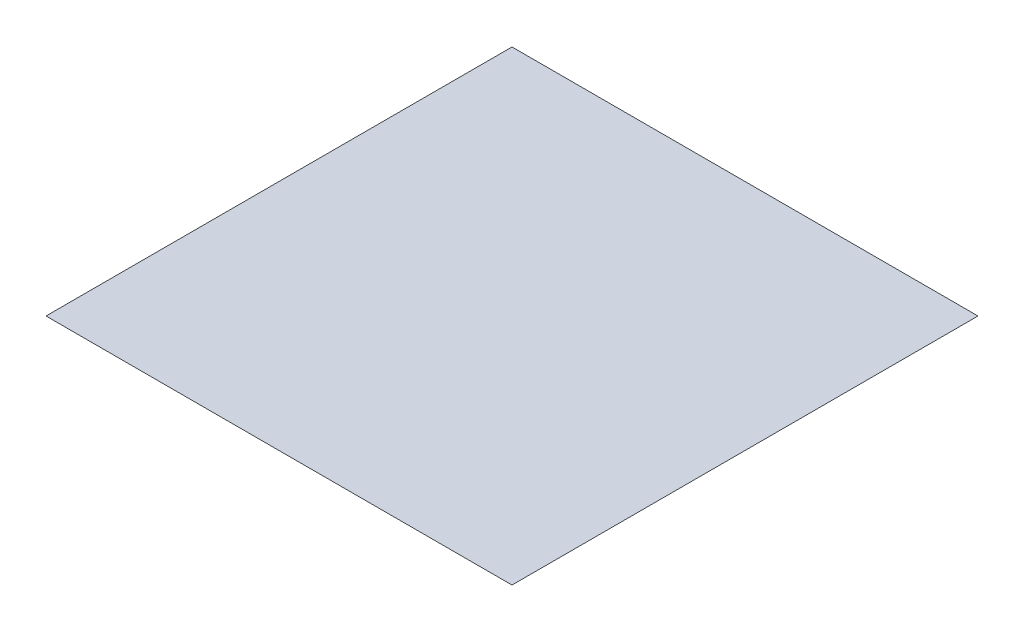
from build123d import *


with BuildPart() as part:
    # 草图5 → 放样1 section 0
    with BuildSketch(Plane(origin=(0, 100, 0), x_dir=(-1, 0, 0), z_dir=(0, -1, 0))):
        with BuildLine():
            Line((165.564800674, -165.564800674), (-165.564800674, -165.564800674))
            Line((-165.564800674, -165.564800674), (-165.564800674, 165.564800674))
            Line((-165.564800674, 165.564800674), (165.564800674, 165.564800674))
            Line((165.564800674, 165.564800674), (165.564800674, -165.564800674))
        make_face()
    # 草图1 → 放样1 section 1
    with BuildSketch(Plane(origin=(0, 0, 0), x_dir=(1, 0, 0), z_dir=(0, 1, 0))):
        with BuildLine():
            Line((-22.75, 22.75), (22.75, 22.75))
            Line((22.75, 22.75), (22.75, -22.75))
            Line((22.75, -22.75), (-22.75, -22.75))
            Line((-22.75, -22.75), (-22.75, 22.75))
        make_face()
    loft()


solid = part.part
